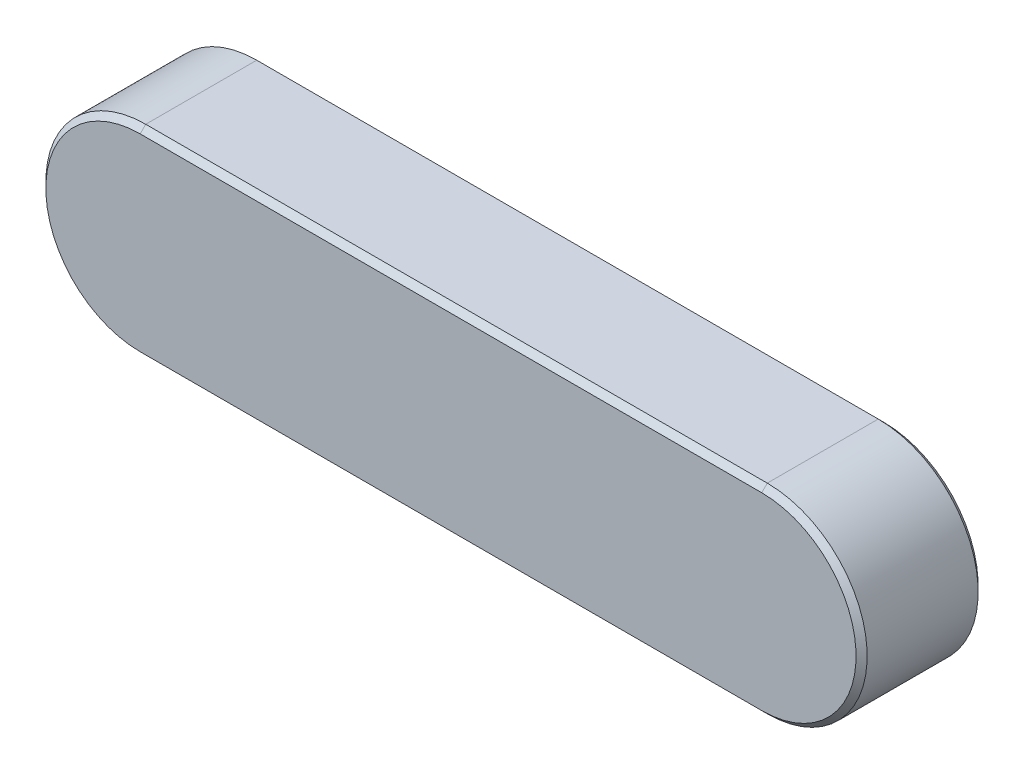
SolidWorks part; units mm, degrees
material "普通碳钢"
ref_plane "Front Plane" through (0, 0, 0) normal (0, 0, 1) x (1, 0, 0)
ref_plane "Top Plane" through (0, 0, 0) normal (0, 1, 0) x (1, 0, 0)
ref_plane "Right Plane" through (0, 0, 0) normal (1, 0, 0) x (0, 0, -1)
other "Configuration Table"
sketch "Sketch1" plane through (0, 0, 0) normal (0, 0, 1) x (1, 0, 0)
  line L0 (0, 0) -> (50, 0) construction
  line L1 (0, 0) -> (0, 9) construction
  line L2 (0, 0) -> (0, -9) construction
  line L3 (0, 0) -> (-50, 0) construction
  line L4 (0, 9) -> (28, 9)
  line L5 (0, -9) -> (28, -9)
  line L6 (0, 9) -> (-28, 9)
  line L7 (0, -9) -> (-28, -9)
  arc A0 (28, 9) -> (28, -9) centre (28, 0) cw
  arc A1 (-28, 9) -> (-28, -9) centre (-28, 0) ccw
  point P12 (-37, 0)
  point P13 (37, 0)
  dimension "D1" = 18
  dimension "D2" = 74
extrude "Boss-Extrude1" add sketch "Sketch1" along normal blind 11
chamfer "Chamfer1" distance 0.5 angle 45 8 edges at (0, -9, 0) (37, 0, 0) (-37, 0, 0) (0, 9, 0) (-37, 0, 11) (0, -9, 11) (37, 0, 11) (0, 9, 11)
